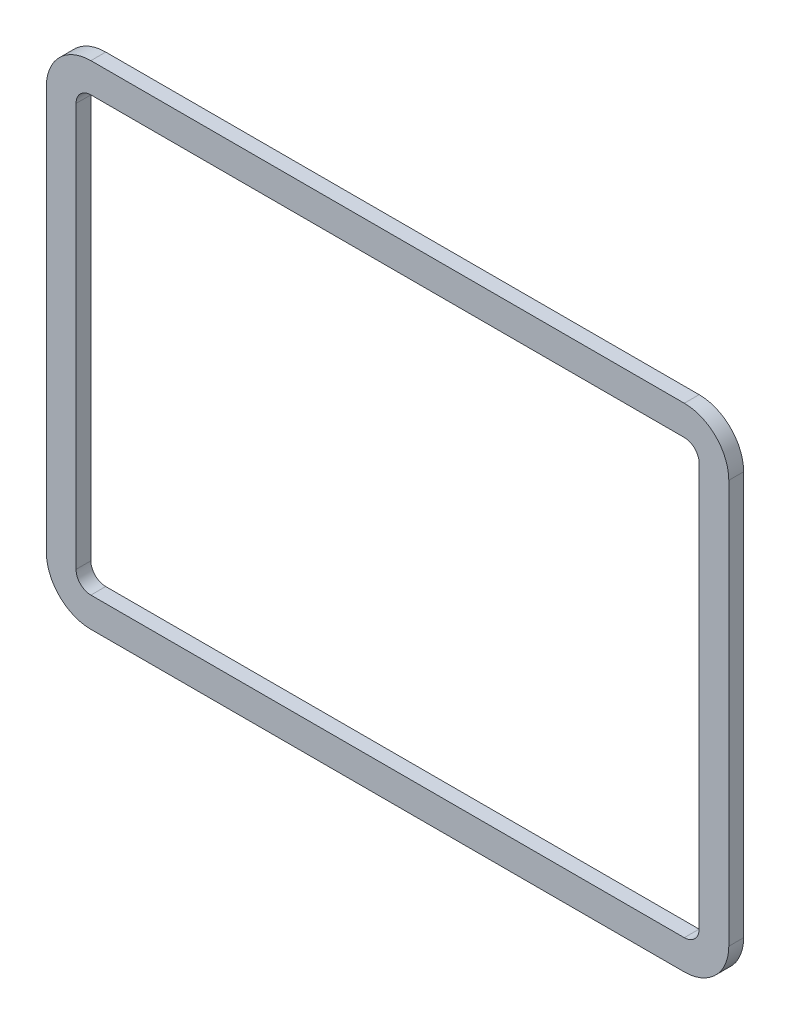
from build123d import *

# Parameters (mm, degrees)
SKETCH1_W           = 230
SKETCH1_H           = 166
SKETCH1_W_2         = 210
SKETCH1_H_2         = 146
BOSS_EXTRUDE1_DEPTH = 5
FILLET1_R           = 5
FILLET2_R           = 15


with BuildPart() as part:
    # Sketch1 → Boss-Extrude1 (new body)
    with BuildSketch(Plane.XY):
        Rectangle(SKETCH1_W, SKETCH1_H)
        Rectangle(SKETCH1_W_2, SKETCH1_H_2, mode=Mode.SUBTRACT)
    extrude(amount=BOSS_EXTRUDE1_DEPTH)

    # Fillet1
    fillet1_edges = [part.edges().sort_by_distance(p)[0] for p in [
        (-105, 73, 2.5),
        (-105, -73, 2.5),
        (105, -73, 2.5),
        (105, 73, 2.5),
    ]]
    fillet(fillet1_edges, radius=FILLET1_R)

    # Fillet2
    fillet2_edges = [part.edges().sort_by_distance(p)[0] for p in [
        (-115, 83, 2.5),
        (115, 83, 2.5),
        (115, -83, 2.5),
        (-115, -83, 2.5),
    ]]
    fillet(fillet2_edges, radius=FILLET2_R)


solid = part.part
